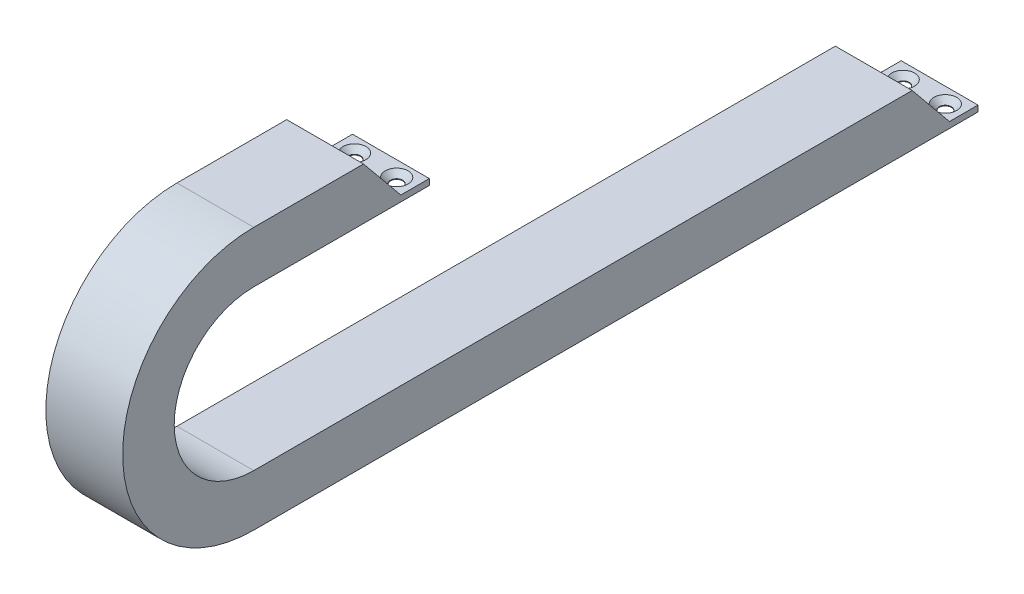
SolidWorks part; units mm, degrees
ref_plane "Front Plane" through (0, 0, 0) normal (0, 0, 1) x (1, 0, 0)
ref_plane "Top Plane" through (0, 0, 0) normal (0, 1, 0) x (1, 0, 0)
ref_plane "Right Plane" through (0, 0, 0) normal (1, 0, 0) x (0, 0, -1)
sketch "Section Size" plane through (0, 0, 0) normal (0, 0, 1) x (1, 0, 0)
  line L0 (-12.5, -9) -> (12.5, 9) construction
  line L1 (-12.5, 9) -> (12.5, 9)
  line L2 (-12.5, 9) -> (-12.5, -9)
  line L3 (-12.5, -9) -> (12.5, -9)
  line L4 (12.5, 9) -> (12.5, -9)
  line L5 (-17.5, 11.75) -> (17.5, -11.75) construction
  line L6 (-17.5, 11.75) -> (17.5, 11.75)
  line L7 (-17.5, 11.75) -> (-17.5, -11.75)
  line L8 (-17.5, -11.75) -> (17.5, -11.75)
  line L9 (17.5, 11.75) -> (17.5, -11.75)
  line L11 (12.5, 9) -> (-12.5, 9) construction
  line L12 (12.5, 9) -> (12.5, -9) construction
  line L13 (12.5, -9) -> (-12.5, -9) construction
  line L14 (-12.5, 9) -> (-12.5, -9) construction
  circle A0 centre (9.0278, 6.5) radius 2.5 construction
  circle A1 centre (10, 1.5954) radius 2.5 construction
  circle A2 centre (10, -3.4046) radius 2.5 construction
  circle A3 centre (4.0278, 6.5) radius 2.5 construction
  circle A4 centre (-0.9722, 6.5) radius 2.5 construction
  circle A5 centre (-5.9722, 6.5) radius 2.5 construction
  circle A6 centre (10, -8.4046) radius 2.5 construction
  dimension "D2" = 5
  dimension "D1" = 35
  dimension "Bi" = 25
  dimension "Hi" = 18
  dimension "Ha" = 23.5
sketch "Length Path" plane through (0, 0, 0) normal (1, 0, 0) x (0, 0, -1)
  line L1 (-300, 96) -> (-250, 96)
  line L2 (-300, 0) -> (0, 0)
  arc A0 (-300, 0) -> (-300, 96) centre (-300, 48) cw
  dimension "D1" = 300
  dimension "R" = 48
  dimension "FLG" = 50
sweep "Chain" add profiles "Section Size" path "Length Path"
sketch "Sketch2" plane through (0, 84.25, 0) normal (0, 1, 0) x (1, 0, 0)
  line L1 (-17.5, -250) -> (17.5, -250)
  line L2 (-17.5, -250) -> (-17.5, -220)
  line L3 (-17.5, -220) -> (17.5, -220)
  line L4 (17.5, -250) -> (17.5, -220)
  line L6 (0, -220) -> (0, -250) construction
  line L8 (-17.5, -250) -> (17.5, -250) construction
  line L10 (0, -227) -> (0, -329) construction
  line L12 (-17.5, -300) -> (-17.5, 0) construction
  line L13 (17.5, -300) -> (17.5, -250) construction
  dimension "D1" = 30
  dimension "D2" = 7
extrude "Fitting114.4.12PZ-1" add sketch "Sketch2" along normal up to surface (2.75 mm away) up to face at (0, 87, 275)
sketch "Sketch6" plane through (0, -11.75, 0) normal (0, -1, 0) x (1, 0, 0)
  line L1 (-17.5, 0) -> (17.5, 0)
  line L2 (-17.5, 0) -> (-17.5, -30)
  line L3 (-17.5, -30) -> (17.5, -30)
  line L4 (17.5, 0) -> (17.5, -30)
  line L7 (0, 0) -> (0, -30) construction
  line L12 (0, -15) -> (0, -23) construction
  dimension "D1" = 30
  dimension "D2" = 7
  dimension "D3" = 8
extrude "Fitting114.4.12PZ-2" add sketch "Sketch6" against normal up to surface (2.75 mm away) up to face at (0, -9, 150)
sketch "Sketch9" plane through (17.5, 0, 0) normal (1, 0, 0) x (0, 0, -1)
  line L0 (-250, 107.75) -> (-233, 87)
  line L1 (-250, 107.75) -> (-250, 87) construction
  line L2 (-220, 87) -> (-250, 87) construction
  dimension "D1" = 17
rib "E" sketch "Sketch9" sketch "Sketch9" thickness 4.1 extrusion direction parallel to sketch draft on no parameters "D1"=4.1
sketch "Sketch10" plane through (17.5, 0, 0) normal (1, 0, 0) x (0, 0, -1)
  line L0 (17, -9) -> (0, 11.75)
  line L3 (30, -9) -> (0, -9) construction
  line L4 (0, -9) -> (0, 11.75) construction
  dimension "D1" = 17
rib "Z" sketch "Sketch10" sketch "Sketch10" thickness 4.1 extrusion direction parallel to sketch draft on no parameters "D1"=4.1
mirror "Drag" about plane through (0, 0, 0) normal (1, 0, 0) of "Z", "E"
sketch "Sketch15" plane through (0, 0, 0) normal (0, 0, -1) x (-1, 0, 0)
  line L0 (-12.5, -9) -> (-12.5, 105) construction
  line L1 (17.5, -9) -> (-17.5, -9) construction
  circle A0 centre (-10.5, -7) radius 2
  circle A1 centre (-6.5, -7) radius 2
  circle A2 centre (-2.5, -7) radius 2
  circle A3 centre (1.5, -7) radius 2
  circle A4 centre (-10.5, -3) radius 2
  circle A5 centre (-6.5, -3) radius 2
  circle A6 centre (-2.5, -3) radius 2
  circle A7 centre (1.5, -3) radius 2
  dimension "D1" = 4
  dimension "D2" = 4
  dimension "D3" = 4
sketch "Sketch16" plane through (0, -9, 0) normal (0, 1, 0) x (1, 0, 0)
  line L0 (0, 30) -> (0, 13) construction
  line L1 (-17.5, 30) -> (17.5, 30) construction
  line L3 (9.6, 23) -> (-9.6, 23) construction
  dimension "D1" = 10
  dimension "D2" = 7
  dimension "D3" = 19.2
hole_wizard "M5 Flat Head Screw Countersink1" positions "3D Sketch1" profile "Sketch17" countersink size "M5" standard "ISO" end condition through all
sketch3d "3D Sketch1"
  point P0 (-9.6, -9, -23)
  point P3 (0, -9, -13)
  point P6 (9.6, -9, -23)
sketch "Sketch17" plane through (-9.6, -9, -23) normal (1, 0, 0) x (0, 0, 1)
  line L0 (0, 0) -> (0, 2.75)
  line L1 (0, 2.75) -> (2.75, 2.75)
  line L2 (2.75, 2.75) -> (2.75, 2.45)
  line L3 (2.75, 2.45) -> (5.2, 0)
  line L5 (5.2, 0) -> (0, 0)
  line L6 (-2.75, 2.45) -> (-5.2, 0) construction
  line L11 (0, -6.35) -> (0, 107.95) construction
  dimension "貫穿孔直徑" = 5.5
  dimension "貫穿孔深度" = 2.75
  dimension "近端錐孔直徑" = 10.4
  dimension "近端錐孔角度" = 90
sketch "Sketch18" plane through (0, 87, 0) normal (0, 1, 0) x (1, 0, 0)
  line L0 (0, -220) -> (0, -237) construction
  line L1 (-17.5, -220) -> (17.5, -220) construction
  line L2 (-17.5, -220) -> (17.5, -220) construction
  line L3 (-9.6, -227) -> (9.6, -227) construction
  dimension "D1" = 7
  dimension "D2" = 10
  dimension "D3" = 19.2
hole_wizard "M5 Flat Head Screw Countersink2" positions "3D Sketch2" profile "Sketch20" countersink size "M5" standard "ISO"
sketch3d "3D Sketch2"
  point P0 (-9.6, 87, 227)
  point P3 (0, 87, 237)
  point P6 (9.6, 87, 227)
sketch "Sketch20" plane through (-9.6, 87, 227) normal (1, 0, 0) x (0, 0, 1)
  line L0 (0, 0) -> (0, 36.6524)
  line L1 (0, 36.6524) -> (2.75, 35)
  line L2 (2.75, 35) -> (2.75, 2.45)
  line L3 (2.75, 2.45) -> (5.2, 0)
  line L5 (5.2, 0) -> (0, 0)
  line L6 (-2.75, 2.45) -> (-5.2, 0) construction
  line L10 (0, 36.6524) -> (-2.75, 35) construction
  line L11 (0, -6.35) -> (0, 107.95) construction
  dimension "鑽孔直徑" = 5.5
  dimension "鑽孔深度" = 35
  dimension "近端錐孔直徑" = 10.4
  dimension "近端錐孔角度" = 90
  dimension "導頭角度" = 118
